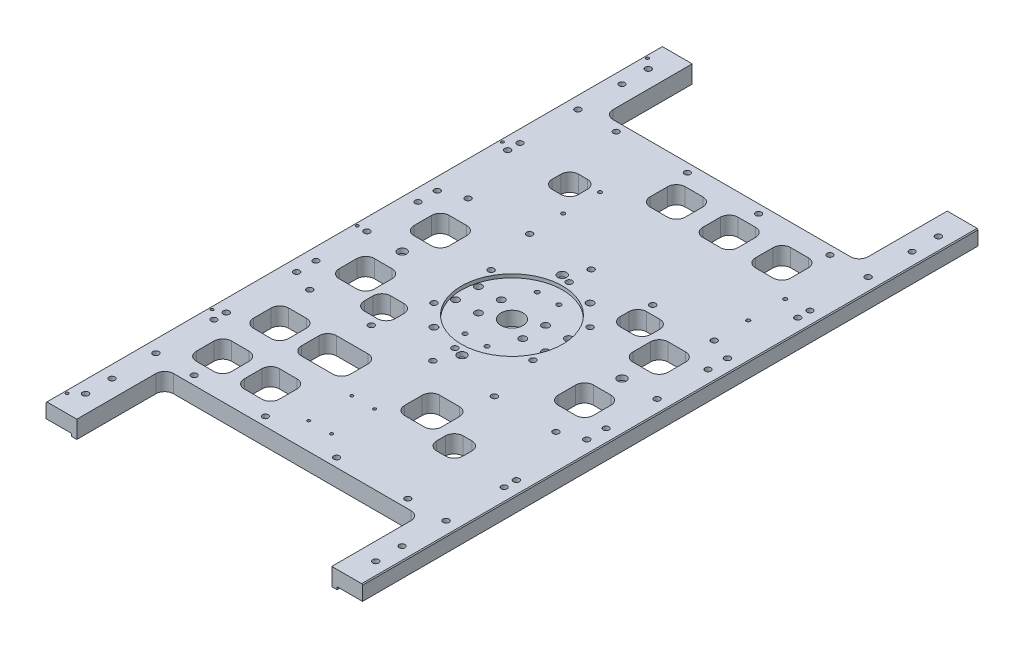
SolidWorks part; units mm, degrees
ref_plane "前视基准面" through (0, 0, 0) normal (0, 0, 1) x (1, 0, 0)
ref_plane "上视基准面" through (0, 0, 0) normal (0, 1, 0) x (1, 0, 0)
ref_plane "右视基准面" through (0, 0, 0) normal (1, 0, 0) x (0, 0, -1)
ref_plane "基准面4" through (0, 0, 0) normal (0, -1, 0) x (1, 0, 0)
sketch "草图1" plane through (0, 0, 0) normal (0, -1, 0) x (1, 0, 0)
  line L0 (180, 350) -> (-180, 350)
  line L1 (-180, 350) -> (-180, -350)
  line L2 (-180, -350) -> (180, -350)
  line L3 (180, -350) -> (180, 350)
extrude "凸台-拉伸1" add sketch "草图1" against normal blind 20
sketch "草图2" plane through (0, 20, 0) normal (0, 1, 0) x (-1, 0, 0)
  line L0 (-145, 350) -> (-145, 250)
  line L1 (-145, 250) -> (145, 250)
  line L2 (145, 250) -> (145, 350)
  line L3 (145, 350) -> (-145, 350)
extrude "切除-拉伸1" cut sketch "草图2" against normal through all
sketch "草图3" plane through (0, 0, 350) normal (0, 0, 1) x (1, 0, 0)
  line L0 (-151, 0) -> (-151, 3)
  line L1 (-151, 3) -> (-180, 3)
  line L2 (-180, 3) -> (-180, 0)
  line L3 (-180, 0) -> (-151, 0)
extrude "切除-拉伸2" cut sketch "草图3" against normal through all
sketch "草图4" plane through (0, 0, 350) normal (0, 0, 1) x (1, 0, 0)
  line L0 (151, 3) -> (151, 0)
  line L1 (151, 0) -> (180, 0)
  line L2 (180, 0) -> (180, 3)
  line L3 (180, 3) -> (151, 3)
extrude "切除-拉伸3" cut sketch "草图4" against normal through all
sketch "草图5" plane through (0, 20, 0) normal (0, 1, 0) x (-1, 0, 0)
  line L0 (145, -350) -> (145, -250)
  line L1 (145, -250) -> (-145, -250)
  line L2 (-145, -250) -> (-145, -350)
  line L3 (-145, -350) -> (145, -350)
extrude "切除-拉伸4" cut sketch "草图5" against normal through all
sketch "草图6" plane through (0, 0, 0) normal (0, -1, 0) x (1, 0, 0)
  line L0 (81.993, -185) -> (81.993, -225)
  line L1 (81.993, -225) -> (121.993, -225)
  line L2 (121.993, -225) -> (121.993, -185)
  line L3 (121.993, -185) -> (81.993, -185)
extrude "切除-拉伸5" cut sketch "草图6" against normal through all
sketch "草图7" plane through (0, 0, 0) normal (0, -1, 0) x (1, 0, 0)
  line L0 (61.993, -185) -> (21.993, -185)
  line L1 (21.993, -185) -> (21.993, -225)
  line L2 (21.993, -225) -> (61.993, -225)
  line L3 (61.993, -225) -> (61.993, -185)
extrude "切除-拉伸6" cut sketch "草图7" against normal through all
sketch "草图8" plane through (0, 0, 0) normal (0, -1, 0) x (1, 0, 0)
  line L0 (105, -22.5) -> (105, -62.5)
  line L1 (105, -62.5) -> (145, -62.5)
  line L2 (145, -62.5) -> (145, -22.5)
  line L3 (145, -22.5) -> (105, -22.5)
extrude "切除-拉伸7" cut sketch "草图8" against normal through all
sketch "草图9" plane through (0, 0, 0) normal (0, -1, 0) x (1, 0, 0)
  line L0 (1.993, -185) -> (-38.007, -185)
  line L1 (-38.007, -185) -> (-38.007, -225)
  line L2 (-38.007, -225) -> (1.993, -225)
  line L3 (1.993, -225) -> (1.993, -185)
extrude "切除-拉伸8" cut sketch "草图9" against normal through all
sketch "草图10" plane through (0, 0, 0) normal (0, -1, 0) x (1, 0, 0)
  line L0 (105, 62.5) -> (105, 22.5)
  line L1 (105, 22.5) -> (145, 22.5)
  line L2 (145, 22.5) -> (145, 62.5)
  line L3 (145, 62.5) -> (105, 62.5)
extrude "切除-拉伸9" cut sketch "草图10" against normal through all
sketch "草图11" plane through (0, 0, 0) normal (0, -1, 0) x (1, 0, 0)
  line L0 (-104, 62.5) -> (-144, 62.5)
  line L1 (-144, 62.5) -> (-144, 22.5)
  line L2 (-144, 22.5) -> (-104, 22.5)
  line L3 (-104, 22.5) -> (-104, 62.5)
extrude "切除-拉伸10" cut sketch "草图11" against normal through all
sketch "草图12" plane through (0, 0, 0) normal (0, -1, 0) x (1, 0, 0)
  line L0 (-144, -62.5) -> (-104, -62.5)
  line L1 (-104, -62.5) -> (-104, -22.5)
  line L2 (-104, -22.5) -> (-144, -22.5)
  line L3 (-144, -22.5) -> (-144, -62.5)
extrude "切除-拉伸11" cut sketch "草图12" against normal through all
sketch "草图13" plane through (0, 0, 0) normal (0, -1, 0) x (1, 0, 0)
  line L0 (-89.5, 225) -> (-89.5, 185)
  line L1 (-89.5, 185) -> (-49.5, 185)
  line L2 (-49.5, 185) -> (-49.5, 225)
  line L3 (-49.5, 225) -> (-89.5, 225)
extrude "切除-拉伸12" cut sketch "草图13" against normal through all
sketch "草图14" plane through (0, 0, 0) normal (0, -1, 0) x (1, 0, 0)
  line L0 (27.8007, 160) -> (27.8007, 120)
  line L1 (27.8007, 120) -> (70.0923, 120)
  line L2 (70.0923, 120) -> (70.0923, 160)
  line L3 (70.0923, 160) -> (27.8007, 160)
extrude "切除-拉伸13" cut sketch "草图14" against normal through all
sketch "草图15" plane through (0, 0, 0) normal (0, -1, 0) x (1, 0, 0)
  line L0 (-33.7573, 160) -> (-89.5, 160)
  line L1 (-89.5, 160) -> (-89.5, 120)
  line L2 (-89.5, 120) -> (-33.7573, 120)
  line L3 (-33.7573, 120) -> (-33.7573, 160)
extrude "切除-拉伸14" cut sketch "草图15" against normal through all
sketch "草图16" plane through (0, 0, 0) normal (0, -1, 0) x (1, 0, 0)
  line L0 (-104, 225) -> (-144, 225)
  line L1 (-144, 225) -> (-144, 185)
  line L2 (-144, 185) -> (-104, 185)
  line L3 (-104, 185) -> (-104, 225)
extrude "切除-拉伸15" cut sketch "草图16" against normal through all
sketch "草图17" plane through (0, 0, 0) normal (0, -1, 0) x (1, 0, 0)
  line L0 (-104, 160) -> (-144, 160)
  line L1 (-144, 160) -> (-144, 120)
  line L2 (-144, 120) -> (-104, 120)
  line L3 (-104, 120) -> (-104, 160)
extrude "切除-拉伸16" cut sketch "草图17" against normal through all
sketch "草图18" plane through (0, 0, 0) normal (0, -1, 0) x (1, 0, 0)
  line L0 (-81, -146.668) -> (-111, -146.668)
  line L1 (-111, -146.668) -> (-111, -176.668)
  line L2 (-111, -176.668) -> (-81, -176.668)
  line L3 (-81, -176.668) -> (-81, -146.668)
extrude "切除-拉伸17" cut sketch "草图18" against normal through all
sketch "草图19" plane through (0, 0, 0) normal (0, -1, 0) x (1, 0, 0)
  line L0 (81, 146.668) -> (111, 146.668)
  line L1 (111, 146.668) -> (111, 176.668)
  line L2 (111, 176.668) -> (81, 176.668)
  line L3 (81, 176.668) -> (81, 146.668)
extrude "切除-拉伸18" cut sketch "草图19" against normal through all
sketch "草图20" plane through (0, 0, 0) normal (0, -1, 0) x (1, 0, 0)
  line L0 (63, -80) -> (98, -80)
  line L1 (98, -80) -> (98, -50)
  line L2 (98, -50) -> (63, -50)
  line L3 (63, -50) -> (63, -80)
extrude "切除-拉伸19" cut sketch "草图20" against normal through all
sketch "草图21" plane through (0, 20, 0) normal (0, 1, 0) x (-1, 0, 0)
  line L0 (63, 80) -> (63, 50)
  line L1 (63, 50) -> (98, 50)
  line L2 (98, 50) -> (98, 80)
  line L3 (98, 80) -> (63, 80)
extrude "切除-拉伸20" cut sketch "草图21" against normal through all
sketch "草图22" plane through (0, 0, 0) normal (0, -1, 0) x (1, 0, 0)
  line L0 (-21.2, -41) -> (-21.2, 41)
  line L1 (-21.2, 41) -> (-55.2, 41)
  line L2 (-55.2, 41) -> (-55.2, -41)
  line L3 (-55.2, -41) -> (-21.2, -41)
extrude "切除-拉伸21" cut sketch "草图22" against normal blind 5
sketch "草图23" plane through (0, 0, 0) normal (0, -1, 0) x (1, 0, 0)
  line L0 (21.2, 41) -> (21.2, -41)
  line L1 (21.2, -41) -> (55.2, -41)
  line L2 (55.2, -41) -> (55.2, 41)
  line L3 (55.2, 41) -> (21.2, 41)
extrude "切除-拉伸22" cut sketch "草图23" against normal blind 5
sketch "草图24" plane through (0, 0, 0) normal (0, -1, 0) x (1, 0, 0)
  line L0 (55, 225) -> (-40, 225)
  line L1 (-40, 225) -> (-40, 165)
  line L2 (-40, 165) -> (55, 165)
  line L3 (55, 165) -> (55, 225)
extrude "切除-拉伸23" cut sketch "草图24" against normal blind 12
sketch "草图25" plane through (0, 0, 0) normal (0, -1, 0) x (1, 0, 0)
  line L0 (145, -100) -> (-75, -100)
  line L1 (-75, -100) -> (-75, -180)
  line L2 (-75, -180) -> (145, -180)
  line L3 (145, -180) -> (145, -100)
extrude "切除-拉伸24" cut sketch "草图25" against normal blind 12
ref_plane "基准面5" through (0, 0, -0.1312) normal (0, 0, -1) x (-1, 0, 0)
sketch "草图26" plane through (0, 0, -0.1312) normal (0, 0, -1) x (-1, 0, 0)
  line L0 (-130, 0) -> (-125, 0)
  line L1 (-125, 0) -> (-125, 20)
  line L2 (-125, 20) -> (-130, 20)
  line L3 (-130, 20) -> (-130, 14.6)
  line L4 (-130, 14.6) -> (-127.75, 14.6)
  line L5 (-127.75, 14.6) -> (-127.75, 6)
  line L6 (-127.75, 6) -> (-130, 6)
  line L7 (-130, 6) -> (-130, 0)
  line L8 (-125, 0) -> (-125, 20) construction
revolve "切除-旋转1" cut sketch "草图26" angle 360 about L8
sketch "草图27" plane through (0, 0, -0.1312) normal (0, 0, -1) x (-1, 0, 0)
  line L0 (120, 0) -> (125, 0)
  line L1 (125, 0) -> (125, 20)
  line L2 (125, 20) -> (120, 20)
  line L3 (120, 20) -> (120, 14.6)
  line L4 (120, 14.6) -> (122.25, 14.6)
  line L5 (122.25, 14.6) -> (122.25, 6)
  line L6 (122.25, 6) -> (120, 6)
  line L7 (120, 6) -> (120, 0)
  line L8 (125, 0) -> (125, 20) construction
revolve "切除-旋转2" cut sketch "草图27" angle 360 about L8
ref_plane "基准面6" through (0, 0, -68.1312) normal (0, 0, -1) x (-1, 0, 0)
sketch "草图28" plane through (0, 0, -68.1312) normal (0, 0, -1) x (-1, 0, 0)
  line L0 (6, 0) -> (11, 0)
  line L1 (11, 0) -> (11, 20)
  line L2 (11, 20) -> (6, 20)
  line L3 (6, 20) -> (6, 14.6)
  line L4 (6, 14.6) -> (8.25, 14.6)
  line L5 (8.25, 14.6) -> (8.25, 6)
  line L6 (8.25, 6) -> (6, 6)
  line L7 (6, 6) -> (6, 0)
  line L8 (11, 0) -> (11, 20) construction
revolve "切除-旋转3" cut sketch "草图28" angle 360 about L8
ref_plane "基准面7" through (0, 0, 67.8688) normal (0, 0, -1) x (-1, 0, 0)
sketch "草图29" plane through (0, 0, 67.8688) normal (0, 0, -1) x (-1, 0, 0)
  line L0 (-16, 0) -> (-11, 0)
  line L1 (-11, 0) -> (-11, 20)
  line L2 (-11, 20) -> (-16, 20)
  line L3 (-16, 20) -> (-16, 14.6)
  line L4 (-16, 14.6) -> (-13.75, 14.6)
  line L5 (-13.75, 14.6) -> (-13.75, 6)
  line L6 (-13.75, 6) -> (-16, 6)
  line L7 (-16, 6) -> (-16, 0)
  line L8 (-11, 0) -> (-11, 20) construction
revolve "切除-旋转4" cut sketch "草图29" angle 360 about L8
hole_wizard "Ø4.2 (4.2) 直径孔1" positions "草图31" profile "草图30" hole size "Ø4.2" standard "ANSI Metric"
sketch "草图31" plane through (0, 12, 0) normal (0, -1, 0) x (-1, 0, 0)
  point P0 (71, 171.2)
  point P1 (71, 129.2)
  point P2 (-139.5, 129.2)
  point P3 (-139.5, 171.2)
sketch "草图30" plane through (-71, 12, -171.2) normal (1, 0, 0) x (0, 0, -1)
  line L0 (0, 0) -> (0, 8)
  line L1 (0, 8) -> (2.1, 8)
  line L2 (2.1, 8) -> (2.1, 0)
  line L5 (2.1, 0) -> (0, 0)
  line L11 (0, -6.35) -> (0, 107.95) construction
  dimension "通孔孔直径" = 4.2
  dimension "通孔孔深度" = 8
hole_wizard "Ø3.3 (3.3) 直径孔1" positions "草图33" profile "草图32" hole size "Ø3.3" standard "ANSI Metric"
sketch "草图33" plane through (0, 12, 0) normal (0, -1, 0) x (-1, 0, 0)
  point P0 (11.7, -219.5)
  point P1 (-14.3, -219.5)
  point P2 (11.7, -170.5)
  point P3 (-14.3, -170.5)
sketch "草图32" plane through (-11.7, 12, 219.5) normal (1, 0, 0) x (0, 0, -1)
  line L0 (0, 0) -> (0, 8)
  line L1 (0, 8) -> (1.65, 8)
  line L2 (1.65, 8) -> (1.65, 0)
  line L5 (1.65, 0) -> (0, 0)
  line L11 (0, -6.35) -> (0, 107.95) construction
  dimension "通孔孔直径" = 3.3
  dimension "通孔孔深度" = 8
hole_wizard "Ø8.0 (8) 直径孔1" positions "草图35" profile "草图34" hole size "Ø8.0" standard "ANSI Metric"
sketch "草图35" plane through (0, 0, 0) normal (0, -1, 0) x (-1, 0, 0)
  point P0 (-32.5, 56.2917)
  point P1 (32.5, -56.2917)
sketch "草图34" plane through (32.5, 0, -56.2917) normal (1, 0, 0) x (0, 0, -1)
  line L0 (0, 0) -> (0, 20)
  line L1 (0, 20) -> (4, 20)
  line L2 (4, 20) -> (4, 0)
  line L5 (4, 0) -> (0, 0)
  line L11 (0, -6.35) -> (0, 107.95) construction
  dimension "通孔孔直径" = 8
  dimension "通孔孔深度" = 20
hole_wizard "Ø6.8 (6.8) 直径孔1" positions "草图37" profile "草图36" hole size "Ø6.8" standard "ANSI Metric"
sketch "草图37" plane through (0, 20, 0) normal (0, 1, 0) x (1, 0, 0)
  point P0 (-165, -320)
  point P1 (-165, -240)
  point P2 (-165, -160)
  point P3 (-165, -80)
  point P4 (-165, 0)
  point P5 (-165, 80)
  point P6 (-165, 160)
  point P7 (-165, 240)
  point P8 (-165, 320)
  point P9 (165, -320)
  point P10 (165, -240)
  point P11 (165, -160)
  point P12 (165, -80)
  point P13 (165, 0)
  point P14 (165, 80)
  point P15 (165, 160)
  point P16 (165, 240)
  point P17 (165, 320)
sketch "草图36" plane through (-165, 20, 320) normal (1, 0, 0) x (0, 0, 1)
  line L0 (0, 0) -> (0, 20)
  line L1 (0, 20) -> (3.4, 20)
  line L2 (3.4, 20) -> (3.4, 0)
  line L5 (3.4, 0) -> (0, 0)
  line L11 (0, -6.35) -> (0, 107.95) construction
  dimension "通孔孔直径" = 6.8
  dimension "通孔孔深度" = 20
hole_wizard "Ø3.3 (3.3) 直径孔2" positions "草图39" profile "草图38" hole size "Ø3.3" standard "ANSI Metric"
sketch "草图39" plane through (0, 20, 0) normal (0, 1, 0) x (1, 0, 0)
  point P0 (-176, 330)
  point P1 (-176, 165)
  point P2 (-176, 0)
  point P3 (-176, -165)
  point P4 (-176, -330)
sketch "草图38" plane through (-176, 20, -330) normal (1, 0, 0) x (0, 0, 1)
  line L0 (0, 0) -> (0, 11.0914)
  line L1 (0, 11.0914) -> (1.65, 10.1)
  line L2 (1.65, 10.1) -> (1.65, 0)
  line L5 (1.65, 0) -> (0, 0)
  line L10 (0, 11.0914) -> (-1.65, 10.1) construction
  line L11 (0, -6.35) -> (0, 107.95) construction
  dimension "孔直径" = 3.3
  dimension "孔深度" = 10.1
  dimension "导头角度" = 118
hole_wizard "Ø6.8 (6.8) 直径孔2" positions "草图41" profile "草图40" hole size "Ø6.8" standard "ANSI Metric"
sketch "草图41" plane through (0, 20, 0) normal (0, 1, 0) x (1, 0, 0)
  point P0 (140, -90)
  point P1 (70, -90)
  point P2 (0, -90)
  point P3 (-70, -90)
  point P4 (-140, -90)
  point P5 (56.2917, -32.5)
  point P6 (0, -65)
  point P7 (-56.2917, -32.5)
  point P8 (-56.2917, 32.5)
  point P9 (0, 65)
  point P10 (56.2917, 32.5)
  point P11 (140, 90)
  point P12 (70, 90)
  point P13 (0, 90)
  point P14 (-70, 90)
  point P15 (-140, 90)
sketch "草图40" plane through (140, 20, 90) normal (1, 0, 0) x (0, 0, 1)
  line L0 (0, 0) -> (0, 20)
  line L1 (0, 20) -> (3.4, 20)
  line L2 (3.4, 20) -> (3.4, 0)
  line L5 (3.4, 0) -> (0, 0)
  line L11 (0, -6.35) -> (0, 107.95) construction
  dimension "通孔孔直径" = 6.8
  dimension "通孔孔深度" = 20
hole_wizard "M6 六角头螺栓的柱形沉头孔1" positions "草图43" profile "草图42" counterbore size "M6" standard "ANSI Metric"
sketch "草图43" plane through (0, 0, 0) normal (0, -1, 0) x (-1, 0, 0)
  point P0 (40.5, -240)
  point P1 (-40.5, -240)
  point P2 (-121.5, -240)
  point P3 (121.5, -240)
  point P4 (-121.5, 240)
  point P5 (-40.5, 240)
  point P6 (40.5, 240)
  point P7 (121.5, 240)
sketch "草图42" plane through (-40.5, 0, 240) normal (1, 0, 0) x (0, 0, -1)
  line L0 (0, 0) -> (0, 20)
  line L1 (0, 20) -> (3.3, 20)
  line L3 (3.3, 20) -> (3.3, 6.4)
  line L4 (3.3, 6.4) -> (5.5, 6.4)
  line L5 (5.5, 6.4) -> (5.5, 0)
  line L7 (5.5, 0) -> (0, 0)
  line L11 (0, -6.35) -> (0, 107.95) construction
  dimension "通孔孔直径" = 6.6
  dimension "通孔孔深度" = 20
  dimension "柱形沉头孔直径" = 11
  dimension "柱形沉头孔深度" = 6.4
hole_wizard "M6 六角头螺栓的柱形沉头孔2" positions "草图45" profile "草图44" counterbore size "M6" standard "ANSI Metric"
sketch "草图45" plane through (0, 3, 0) normal (0, -1, 0) x (-1, 0, 0)
  point P0 (165, 58)
  point P1 (165, 174)
  point P2 (165, 290)
  point P3 (165, -58)
  point P4 (165, -174)
  point P5 (165, -290)
  point P6 (-165, -290)
  point P7 (-165, -174)
  point P8 (-165, -58)
  point P9 (-165, 58)
  point P10 (-165, 174)
  point P11 (-165, 290)
sketch "草图44" plane through (-165, 3, -58) normal (1, 0, 0) x (0, 0, -1)
  line L0 (0, 0) -> (0, 17)
  line L1 (0, 17) -> (3.3, 17)
  line L3 (3.3, 17) -> (3.3, 6.4)
  line L4 (3.3, 6.4) -> (5.5, 6.4)
  line L5 (5.5, 6.4) -> (5.5, 0)
  line L7 (5.5, 0) -> (0, 0)
  line L11 (0, -6.35) -> (0, 107.95) construction
  dimension "通孔孔直径" = 6.6
  dimension "通孔孔深度" = 17
  dimension "柱形沉头孔直径" = 11
  dimension "柱形沉头孔深度" = 6.4
hole_wizard "M24 六角头螺栓的柱形沉头孔1" positions "草图47" profile "草图46" counterbore size "M24" standard "ANSI Metric"
sketch "草图47" plane through (0, 20, 0) normal (0, 1, 0) x (1, 0, 0)
  point P0 (0, 0)
sketch "草图46" plane through (0, 20, 0) normal (1, 0, 0) x (0, 0, 1)
  line L0 (0, 0) -> (0, 20)
  line L1 (0, 20) -> (12.5, 20)
  line L3 (12.5, 20) -> (12.5, 4)
  line L4 (12.5, 4) -> (57.5, 4)
  line L5 (57.5, 4) -> (57.5, 0)
  line L7 (57.5, 0) -> (0, 0)
  line L11 (0, -6.35) -> (0, 107.95) construction
  dimension "通孔孔直径" = 25
  dimension "通孔孔深度" = 20
  dimension "柱形沉头孔直径" = 115
  dimension "柱形沉头孔深度" = 4
hole_wizard "Ø5.0 (5) 直径孔1" positions "草图49" profile "草图48" hole size "Ø5.0" standard "ANSI Metric"
sketch "草图49" plane through (0, 0, 0) normal (0, -1, 0) x (-1, 0, 0)
  point P0 (-12.3391, 41)
  point P1 (12.3391, 41)
  point P2 (-12.5, -41)
  point P3 (12.5, -41)
sketch "草图48" plane through (12.3391, 0, -41) normal (1, 0, 0) x (0, 0, -1)
  line L0 (0, 0) -> (0, 20)
  line L1 (0, 20) -> (2.5, 20)
  line L2 (2.5, 20) -> (2.5, 0)
  line L5 (2.5, 0) -> (0, 0)
  line L11 (0, -6.35) -> (0, 107.95) construction
  dimension "通孔孔直径" = 5
  dimension "通孔孔深度" = 20
hole_wizard "M4 六角头机械螺钉的柱形沉头孔1" positions "草图51" profile "草图50" counterbore size "M4" standard "ANSI Metric"
sketch "草图51" plane through (0, 16, 0) normal (0, 1, 0) x (1, 0, 0)
  point P0 (-51.2, -13)
  point P1 (-25.2, -13)
  point P2 (-25.2, 13)
  point P3 (-51.2, 13)
  point P4 (51.2, -13)
  point P5 (25.2, -13)
  point P6 (25.2, 13)
  point P7 (51.2, 13)
sketch "草图50" plane through (-51.2, 16, 13) normal (1, 0, 0) x (0, 0, 1)
  line L0 (0, 0) -> (0, 16)
  line L1 (0, 16) -> (2.25, 16)
  line L3 (2.25, 16) -> (2.25, 6)
  line L4 (2.25, 6) -> (4, 6)
  line L5 (4, 6) -> (4, 0)
  line L7 (4, 0) -> (0, 0)
  line L11 (0, -6.35) -> (0, 107.95) construction
  dimension "通孔孔直径" = 4.5
  dimension "通孔孔深度" = 16
  dimension "柱形沉头孔直径" = 8
  dimension "柱形沉头孔深度" = 6
hole_wizard "Ø5.0 (5) 直径孔2" positions "草图53" profile "草图52" hole size "Ø5.0" standard "ANSI Metric"
sketch "草图53" plane through (0, 0, 0) normal (0, -1, 0) x (-1, 0, 0)
  point P0 (-110.1847, -215.5)
  point P1 (-110.1847, -189.5)
  point P2 (-66.1847, -215.5)
  point P3 (-66.1847, -189.5)
  point P4 (110.1847, 215.5)
  point P5 (110.1847, 189.5)
  point P6 (66.1847, 215.5)
  point P7 (66.1847, 189.5)
sketch "草图52" plane through (110.1847, 0, 215.5) normal (1, 0, 0) x (0, 0, -1)
  line L0 (0, 0) -> (0, 16.5022)
  line L1 (0, 16.5022) -> (2.5, 15)
  line L2 (2.5, 15) -> (2.5, 0)
  line L5 (2.5, 0) -> (0, 0)
  line L10 (0, 16.5022) -> (-2.5, 15) construction
  line L11 (0, -6.35) -> (0, 107.95) construction
  dimension "孔直径" = 5
  dimension "孔深度" = 15
  dimension "导头角度" = 118
chamfer "倒角1" distance 1 angle 45 2 edges at (180, 20, 0) (-180, 20, 0)
fillet "圆角1" radius 5 8 edges at (-55.2, 2.5, 41) (-21.2, 2.5, -41) (-55.2, 2.5, -41) (55.2, 2.5, 41) (-21.2, 2.5, 41) (21.2, 2.5, 41) (21.2, 2.5, -41) (55.2, 2.5, -41)
fillet "圆角2" radius 10 76 edges at (111, 10, 146.668) (-89.5, 10, 160) (-89.5, 10, 185) (55, 6, 165) (-144, 10, 160) (55, 6, 225) (-98, 10, 80) (-40, 6, 225) (27.8007, 10, 120) (-40, 6, 165) (-144, 10, 225) (145, 6, -180) (-111, 10, -146.668) (145, 6, -100) (98, 10, -80) (-75, 6, -100) (-145, 10, -250) (-75, 6, -180) (70.0923, 10, 160) (121.993, 10, -225) (-33.7573, 10, 120) (121.993, 10, -185) (-104, 10, 185) (81.993, 10, -185) (-104, 10, 120) (81.993, 10, -225) (-81, 10, -176.668) (21.993, 10, -225) (81, 10, 176.668) (61.993, 10, -225) (63, 10, -50) (61.993, 10, -185) (-63, 10, 50) (21.993, 10, -185) (145, 10, 250) (145, 10, -62.5) (-89.5, 10, 225) (145, 10, -22.5) (70.0923, 10, 120) (105, 10, -22.5) (27.8007, 10, 160) (105, 10, -62.5) (-89.5, 10, 120) (-38.007, 10, -225) (-33.7573, 10, 160) (1.993, 10, -225) (-144, 10, 185) (1.993, 10, -185) (-104, 10, 225) (-38.007, 10, -185) (-144, 10, 120) (145, 10, 22.5) (-104, 10, 160) (145, 10, 62.5) (-111, 10, -176.668) (105, 10, 62.5) (-81, 10, -146.668) (105, 10, 22.5) (111, 10, 176.668) (-144, 10, 22.5) (81, 10, 146.668) (-104, 10, 22.5) (98, 10, -50) (-104, 10, 62.5) (63, 10, -80) (-144, 10, 62.5) (-98, 10, 50) (-144, 10, -22.5) (-63, 10, 80) (-144, 10, -62.5) (-145, 10, 250) (-104, 10, -62.5) (145, 10, -250) (-49.5, 10, 185) (-49.5, 10, 225) (-104, 10, -22.5)
